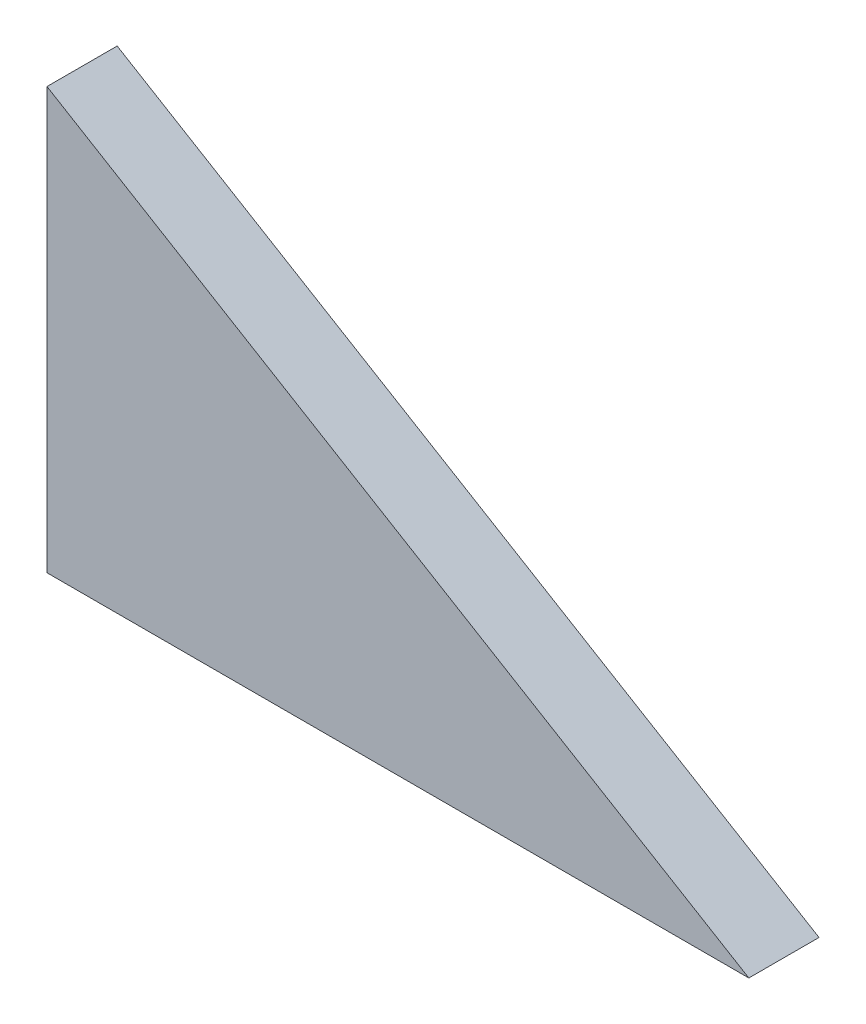
from build123d import *

# Parameters (mm, degrees)
EXTRUDE_1_DEPTH = 5


with BuildPart() as part:
    # 草图1 → 凸台-拉伸1 (new body)
    with BuildSketch(Plane.XY):
        Polygon((0, 0), (0, 30), (50, 0), align=None)
    extrude(amount=EXTRUDE_1_DEPTH)


solid = part.part
